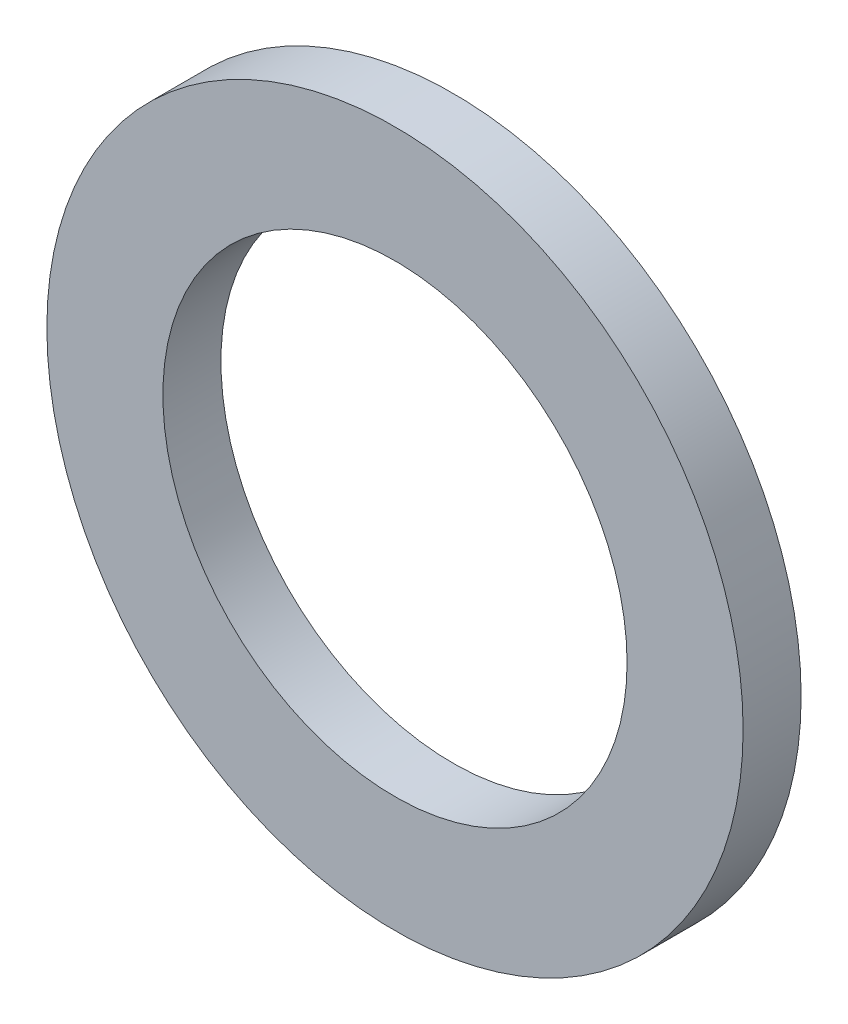
SolidWorks part; units mm, degrees
ref_plane "Front Plane" through (0, 0, 0) normal (0, 0, 1) x (1, 0, 0)
ref_plane "Top Plane" through (0, 0, 0) normal (0, 1, 0) x (1, 0, 0)
ref_plane "Right Plane" through (0, 0, 0) normal (1, 0, 0) x (0, 0, -1)
sketch "Sketch1" plane through (0, 0, 0) normal (0, 0, 1) x (1, 0, 0)
  circle A0 centre (0, 0) radius 40
  circle A1 centre (0, 0) radius 60
  dimension "D1" = 80
  dimension "D2" = 120
extrude "Boss-Extrude1" add sketch "Sketch1" along normal blind 10
